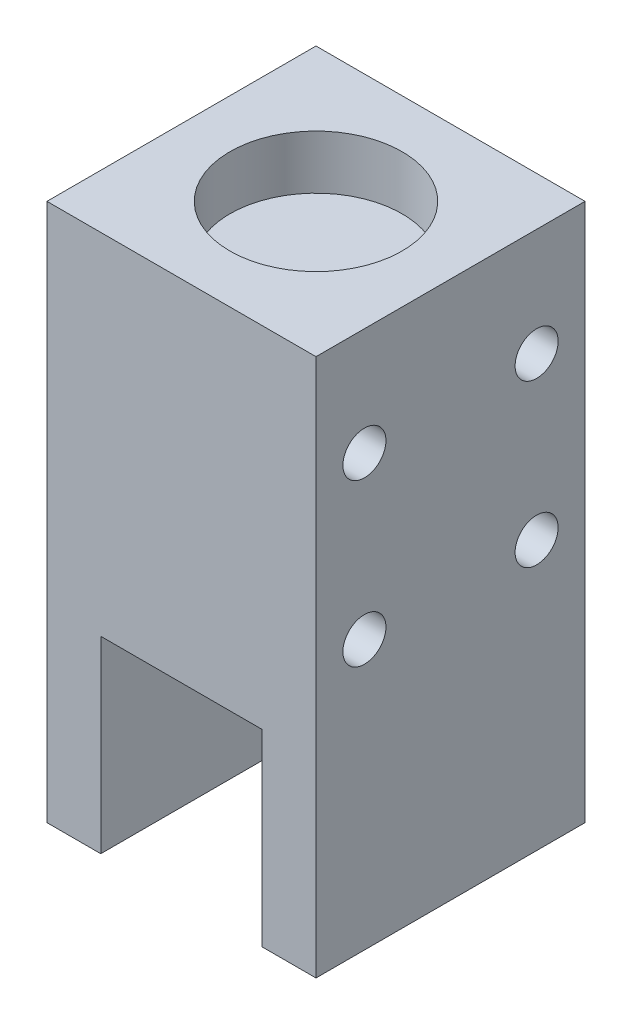
SolidWorks part; units mm, degrees
ref_plane "Front Plane" through (0, 0, 0) normal (0, 0, 1) x (1, 0, 0)
ref_plane "Top Plane" through (0, 0, 0) normal (0, 1, 0) x (1, 0, 0)
ref_plane "Right Plane" through (0, 0, 0) normal (1, 0, 0) x (0, 0, -1)
other "Configuration Table"
sketch "Sketch1" plane through (0, 0, 0) normal (0, 1, 0) x (1, 0, 0)
  line L1 (-25, 25) -> (25, 25)
  line L2 (-25, 25) -> (-25, -25)
  line L3 (-25, -25) -> (25, -25)
  line L4 (25, 25) -> (25, -25)
  line L5 (-25, 25) -> (25, -25) construction
  line L6 (-25, -25) -> (25, 25) construction
  point P0 (0, 0)
  dimension "D1" = 50
  dimension "D2" = 50
extrude "Boss-Extrude1" add sketch "Sketch1" along normal blind 100
sketch "Sketch4" plane through (0, 0, 0) normal (0, -1, 0) x (1, 0, 0)
  line L0 (25, -25) -> (-25, -25) construction
  line L1 (-15, 25) -> (15, 25)
  line L2 (-15, 25) -> (-15, -25)
  line L3 (-15, -25) -> (15, -25)
  line L4 (15, 25) -> (15, -25)
  line L5 (-15, 25) -> (15, -25) construction
  line L6 (-15, -25) -> (15, 25) construction
  point P0 (0, 0)
  dimension "D1" = 30
extrude "Cut-Extrude2" cut sketch "Sketch4" against normal blind 35
sketch "Sketch5" plane through (0, 100, 0) normal (0, 1, 0) x (1, 0, 0)
  line L1 (-22, 22) -> (22, 22)
  line L2 (-22, 22) -> (-22, -22)
  line L3 (-22, -22) -> (22, -22)
  line L4 (22, 22) -> (22, -22)
  line L5 (-22, 22) -> (22, -22) construction
  line L6 (-22, -22) -> (22, 22) construction
  point P0 (0, 0)
  dimension "D1" = 44
  dimension "D2" = 44
sketch "Sketch6" plane through (0, 100, 0) normal (0, 1, 0) x (1, 0, 0)
  circle A0 centre (0, 0) radius 16
  dimension "D1" = 32
extrude "Cut-Extrude3" cut sketch "Sketch6" against normal blind 10
sketch "Sketch8" plane through (-25, 0, 0) normal (-1, 0, 0) x (0, 0, 1)
  line L0 (0, 0) -> (0, 65)
  circle A0 centre (-16, 50) radius 4
  circle A1 centre (-16, 80) radius 4
  circle A2 centre (16, 50) radius 4
  circle A3 centre (16, 80) radius 4
  dimension "D4" = 8
  dimension "D5" = 8
  dimension "D1" = 65
  dimension "D2" = 32
  dimension "D3" = 30
extrude "Cut-Extrude6" cut sketch "Sketch8" against normal blind 10 contours A1 | A3 | A2 | A0
sketch "Sketch9" plane through (25, 0, 0) normal (1, 0, 0) x (0, 0, -1)
  line L0 (0, 0) -> (0, 65)
  circle A0 centre (-16, 80) radius 4
  circle A1 centre (-16, 50) radius 4
  circle A2 centre (16, 50) radius 4
  circle A3 centre (16, 80) radius 4
  dimension "D4" = 8
  dimension "D5" = 8
  dimension "D1" = 65
  dimension "D2" = 32
  dimension "D3" = 30
extrude "Cut-Extrude7" cut sketch "Sketch9" against normal blind 10 contours A0 | A1 | A2 | A3
